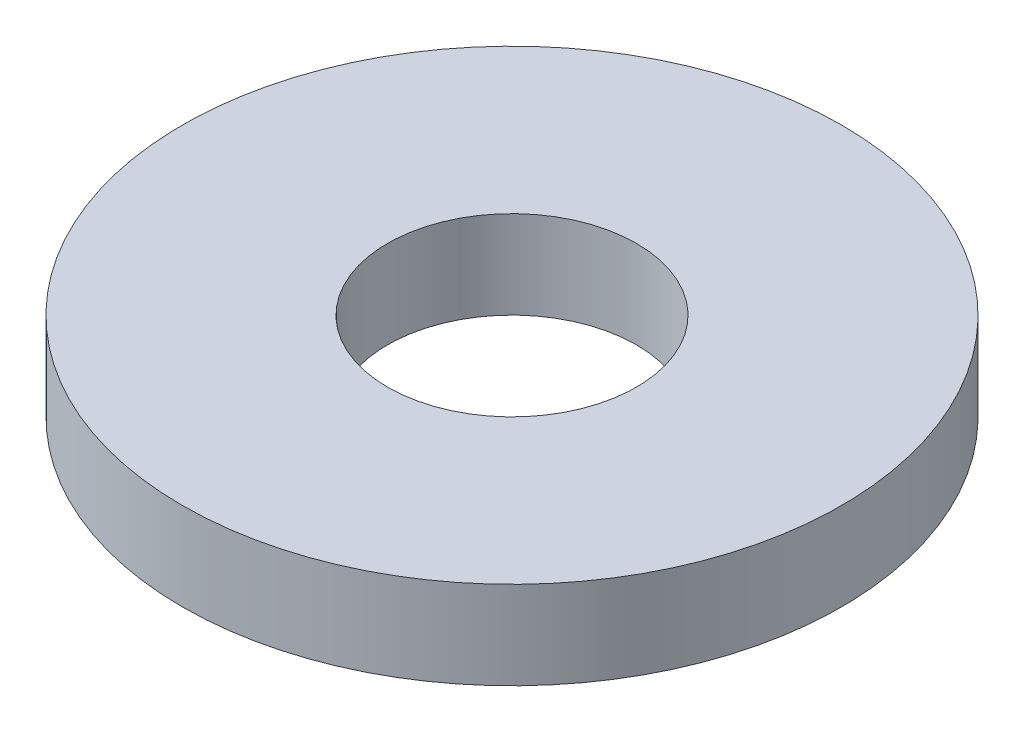
from build123d import *

# Parameters (mm, degrees)
SKETCH1_R           = 22.5
SKETCH1_R_2         = 8.5
BOSS_EXTRUDE1_DEPTH = 6


with BuildPart() as part:
    # Sketch1 → Boss-Extrude1 (new body)
    with BuildSketch(Plane(origin=(0, 0, 0), x_dir=(1, 0, 0), z_dir=(0, 1, 0))):
        with Locations(Location((0, 0, 0), (0, 0, 270))):
            Circle(SKETCH1_R)
        with Locations(Location((0, 0, 0), (0, 0, 270))):
            Circle(SKETCH1_R_2, mode=Mode.SUBTRACT)
    extrude(amount=BOSS_EXTRUDE1_DEPTH)


solid = part.part
